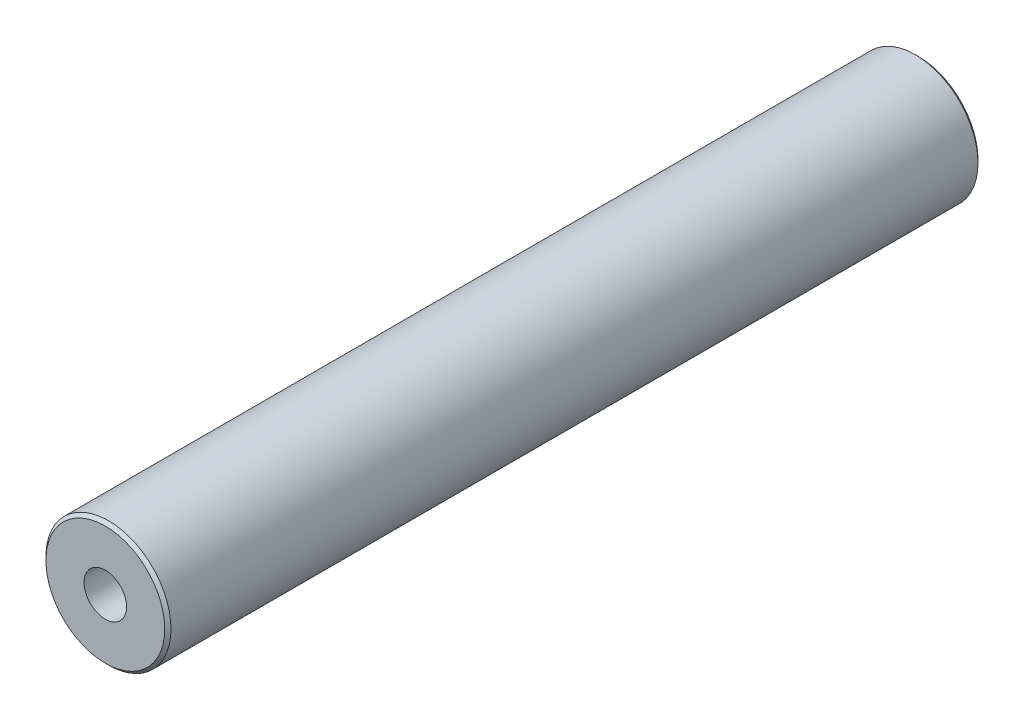
from build123d import *

# Parameters (mm, degrees)
SKETCH_1_R             = 10
EXTRUDE_1_DEPTH        = 130
HOLE_WIZARD_M8_1_D     = 6.8
HOLE_WIZARD_M8_1_DEPTH = 19.75
HOLE_WIZARD_M8_1_TIP   = 2.042926105
HOLE_WIZARD_M8_2_D     = 6.8
HOLE_WIZARD_M8_2_DEPTH = 19.75
HOLE_WIZARD_M8_2_TIP   = 2.042926105
CHAMFER_1_SIZE         = 0.5


with BuildPart() as part:
    # 草图1 → 凸台-拉伸1 (new body)
    with BuildSketch(Plane.XY):
        Circle(SKETCH_1_R)
    extrude(amount=EXTRUDE_1_DEPTH)

    # M8 螺纹孔1
    with Locations(Plane(origin=(0, 0, 0), x_dir=(-1, 0, 0), z_dir=(0, 0, -1))):
        with Locations((0, 0)):
            Hole(HOLE_WIZARD_M8_1_D / 2, depth=HOLE_WIZARD_M8_1_DEPTH)
            with Locations((0, 0, -(HOLE_WIZARD_M8_1_DEPTH + HOLE_WIZARD_M8_1_TIP / 2))):  # 118° drill point
                Cone(0, HOLE_WIZARD_M8_1_D / 2, HOLE_WIZARD_M8_1_TIP, mode=Mode.SUBTRACT)

    # M8 螺纹孔2
    with Locations(Plane.XY.offset(130)):
        with Locations((0, 0)):
            Hole(HOLE_WIZARD_M8_2_D / 2, depth=HOLE_WIZARD_M8_2_DEPTH)
            with Locations((0, 0, -(HOLE_WIZARD_M8_2_DEPTH + HOLE_WIZARD_M8_2_TIP / 2))):  # 118° drill point
                Cone(0, HOLE_WIZARD_M8_2_D / 2, HOLE_WIZARD_M8_2_TIP, mode=Mode.SUBTRACT)

    # 倒角1
    chamfer_1_edges = [part.edges().sort_by_distance(p)[0] for p in [
        (-10, 0, 0),
        (-10, 0, 130),
    ]]
    chamfer(chamfer_1_edges, length=CHAMFER_1_SIZE)


solid = part.part
